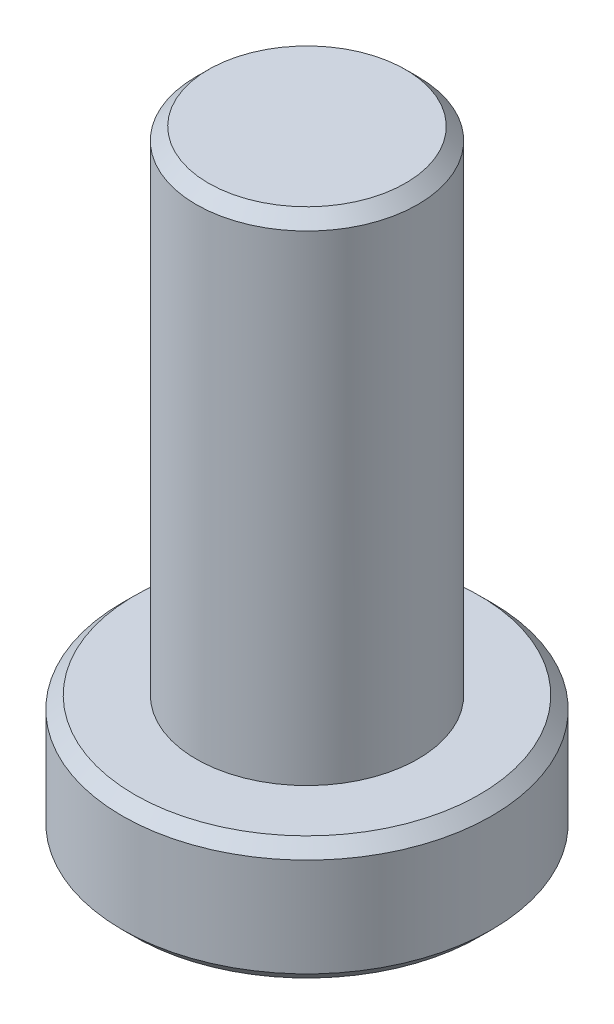
SolidWorks part; units mm, degrees
material "20#"
ref_plane "Front Plane" through (0, 0, 0) normal (0, 0, 1) x (1, 0, 0)
ref_plane "Top Plane" through (0, 0, 0) normal (0, 1, 0) x (1, 0, 0)
ref_plane "Right Plane" through (0, 0, 0) normal (1, 0, 0) x (0, 0, -1)
sketch "Sketch1" plane through (0, 0, 0) normal (1, 0, 0) x (0, 0, -1)
  line L0 (0, 0) -> (0, 25) construction
  line L1 (0, 25) -> (4.5, 25)
  line L2 (4.5, 25) -> (4.5, 5)
  line L3 (4.5, 5) -> (7.5, 5)
  line L4 (7.5, 5) -> (7.5, 0)
  line L5 (7.5, 0) -> (0, 0)
  line L6 (0, 0) -> (0, 25)
  dimension "D1" = 25
  dimension "D2" = 20
  dimension "D3" = 5
  dimension "D4" = 9
  dimension "D5" = 15
revolve "Revolve1" add sketch "Sketch1" angle 360 about L0
chamfer "Chamfer1" distance 0.5 angle 45 3 edges at (0, 0, -7.5) (0, 5, -7.5) (0, 25, -4.5)
